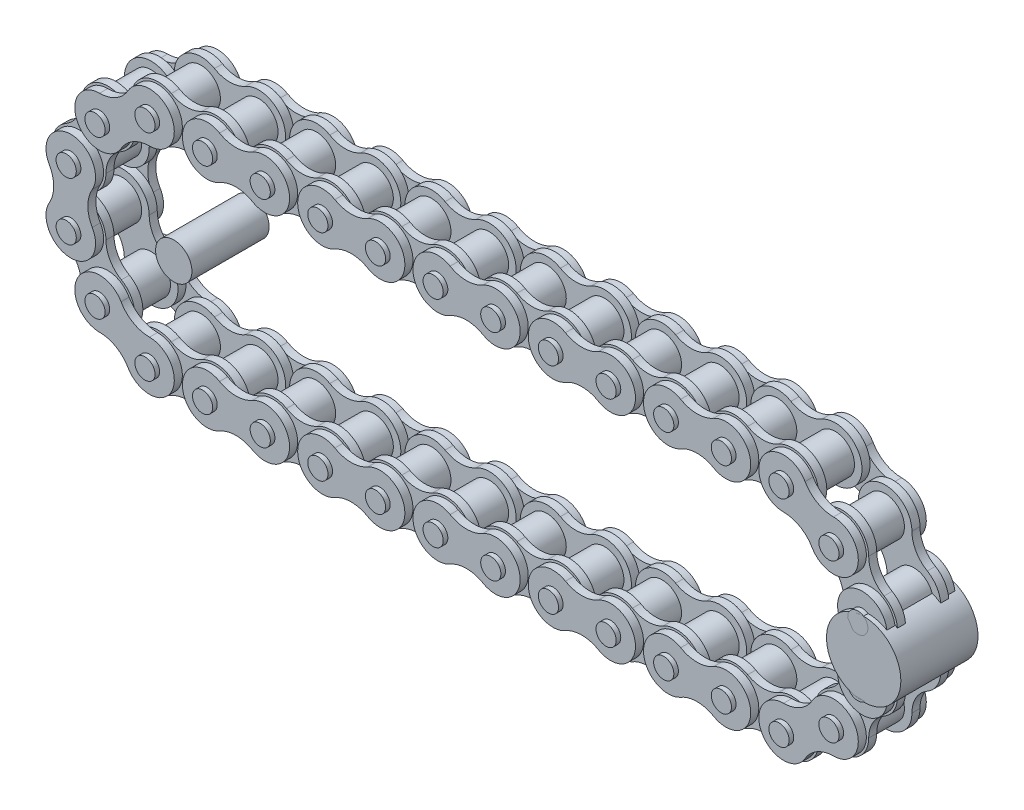
SolidWorks part; units mm, degrees
ref_plane "前视基准面" through (0, 0, 0) normal (0, 0, 1) x (1, 0, 0)
ref_plane "上视基准面" through (0, 0, 0) normal (0, 1, 0) x (1, 0, 0)
ref_plane "右视基准面" through (0, 0, 0) normal (1, 0, 0) x (0, 0, -1)
sketch "草图1" plane through (0, 0, 0) normal (0, 0, 1) x (1, 0, 0)
  circle A0 centre (-23.6985, 6.35) radius 2.225
  circle A1 centre (-23.6985, -6.35) radius 2.225
  circle A2 centre (150.6985, 6.35) radius 2.225
  circle A3 centre (150.6985, -6.35) radius 2.225
  circle A4 centre (-17.3485, 17.3485) radius 2.225
  circle A5 centre (-17.3485, -17.3485) radius 2.225
  circle A6 centre (-6.35, 23.6985) radius 2.225
  circle A7 centre (-6.35, -23.6985) radius 2.225
  circle A8 centre (144.3485, 17.3485) radius 2.225
  circle A9 centre (144.3485, -17.3485) radius 2.225
  circle A10 centre (133.35, 23.6985) radius 2.225
  circle A11 centre (133.35, -23.6985) radius 2.225
  circle A12 centre (6.35, 23.6985) radius 2.225
  circle A13 centre (6.35, -23.6985) radius 2.225
  circle A14 centre (19.05, 23.6985) radius 2.225
  circle A15 centre (19.05, -23.6985) radius 2.225
  circle A16 centre (31.75, 23.6985) radius 2.225
  circle A17 centre (31.75, -23.6985) radius 2.225
  circle A18 centre (44.45, 23.6985) radius 2.225
  circle A19 centre (44.45, -23.6985) radius 2.225
  circle A20 centre (57.15, 23.6985) radius 2.225
  circle A21 centre (57.15, -23.6985) radius 2.225
  circle A22 centre (69.85, 23.6985) radius 2.225
  circle A23 centre (69.85, -23.6985) radius 2.225
  circle A24 centre (82.55, 23.6985) radius 2.225
  circle A25 centre (82.55, -23.6985) radius 2.225
  circle A26 centre (95.25, 23.6985) radius 2.225
  circle A27 centre (95.25, -23.6985) radius 2.225
  circle A28 centre (107.95, 23.6985) radius 2.225
  circle A29 centre (107.95, -23.6985) radius 2.225
  circle A30 centre (120.65, 23.6985) radius 2.225
  circle A31 centre (120.65, -23.6985) radius 2.225
extrude "凸台-拉伸1" add sketch "草图1" along normal blind 8.5 and the other way blind 8.5
sketch "草图2" plane through (0, 0, 0) normal (0, 0, 1) x (1, 0, 0)
  circle A0 centre (-23.6985, 6.35) radius 4.255
  circle A1 centre (-23.6985, -6.35) radius 4.255
  circle A2 centre (150.6985, 6.35) radius 4.255
  circle A3 centre (150.6985, -6.35) radius 4.255
  circle A4 centre (-17.3485, 17.3485) radius 4.255
  circle A5 centre (-17.3485, -17.3485) radius 4.255
  circle A6 centre (-6.35, 23.6985) radius 4.255
  circle A7 centre (-6.35, -23.6985) radius 4.255
  circle A8 centre (144.3485, 17.3485) radius 4.255
  circle A9 centre (144.3485, -17.3485) radius 4.255
  circle A10 centre (133.35, 23.6985) radius 4.255
  circle A11 centre (133.35, -23.6985) radius 4.255
  circle A12 centre (6.35, 23.6985) radius 4.255
  circle A13 centre (6.35, -23.6985) radius 4.255
  circle A14 centre (19.05, 23.6985) radius 4.255
  circle A15 centre (19.05, -23.6985) radius 4.255
  circle A16 centre (31.75, 23.6985) radius 4.255
  circle A17 centre (31.75, -23.6985) radius 4.255
  circle A18 centre (44.45, 23.6985) radius 4.255
  circle A19 centre (44.45, -23.6985) radius 4.255
  circle A20 centre (57.15, 23.6985) radius 4.255
  circle A21 centre (57.15, -23.6985) radius 4.255
  circle A22 centre (69.85, 23.6985) radius 4.255
  circle A23 centre (69.85, -23.6985) radius 4.255
  circle A24 centre (82.55, 23.6985) radius 4.255
  circle A25 centre (82.55, -23.6985) radius 4.255
  circle A26 centre (95.25, 23.6985) radius 4.255
  circle A27 centre (95.25, -23.6985) radius 4.255
  circle A28 centre (107.95, 23.6985) radius 4.255
  circle A29 centre (107.95, -23.6985) radius 4.255
  circle A30 centre (120.65, 23.6985) radius 4.255
  circle A31 centre (120.65, -23.6985) radius 4.255
extrude "凸台-拉伸2" add sketch "草图2" along normal blind 3.875 and the other way blind 3.875
ref_plane "基准面1" through (0, 0, 3.875) normal (0, 0, 1) x (1, 0, 0)
sketch "草图3" plane through (0, 0, 3.875) normal (0, 0, 1) x (1, 0, 0)
  circle A0 centre (-23.6985, 6.35) radius 5.905
  circle A1 centre (-23.6985, -6.35) radius 5.905
  circle A2 centre (150.6985, 6.35) radius 5.905
  circle A3 centre (150.6985, -6.35) radius 5.905
  circle A4 centre (-17.3485, 17.3485) radius 5.905
  circle A5 centre (-17.3485, -17.3485) radius 5.905
  circle A6 centre (-6.35, 23.6985) radius 5.905
  circle A7 centre (-6.35, -23.6985) radius 5.905
  circle A8 centre (144.3485, 17.3485) radius 5.905
  circle A9 centre (144.3485, -17.3485) radius 5.905
  circle A10 centre (133.35, 23.6985) radius 5.905
  circle A11 centre (133.35, -23.6985) radius 5.905
  circle A12 centre (6.35, 23.6985) radius 5.905
  circle A13 centre (6.35, -23.6985) radius 5.905
  circle A14 centre (19.05, 23.6985) radius 5.905
  circle A15 centre (19.05, -23.6985) radius 5.905
  circle A16 centre (31.75, 23.6985) radius 5.905
  circle A17 centre (31.75, -23.6985) radius 5.905
  circle A18 centre (44.45, 23.6985) radius 5.905
  circle A19 centre (44.45, -23.6985) radius 5.905
  circle A20 centre (57.15, 23.6985) radius 5.905
  circle A21 centre (57.15, -23.6985) radius 5.905
  circle A22 centre (69.85, 23.6985) radius 5.905
  circle A23 centre (69.85, -23.6985) radius 5.905
  circle A24 centre (82.55, 23.6985) radius 5.905
  circle A25 centre (82.55, -23.6985) radius 5.905
  circle A26 centre (95.25, 23.6985) radius 5.905
  circle A27 centre (95.25, -23.6985) radius 5.905
  circle A28 centre (107.95, 23.6985) radius 5.905
  circle A29 centre (107.95, -23.6985) radius 5.905
  circle A30 centre (120.65, 23.6985) radius 5.905
  circle A31 centre (120.65, -23.6985) radius 5.905
extrude "凸台-拉伸3" add sketch "草图3" along normal blind 1.775
sketch "草图4" plane through (0, 0, 3.875) normal (0, 0, 1) x (1, 0, 0)
  line L0 (-26.651, 11.4639) -> (-17.7935, 6.35)
  line L1 (-23.2535, 17.3485) -> (-14.396, 12.2346)
  line L2 (-26.651, -11.4639) -> (-17.7935, -6.35)
  line L3 (-23.2535, -17.3485) -> (-14.396, -12.2346)
  line L4 (153.651, 11.4639) -> (144.7935, 6.35)
  line L5 (150.2535, 17.3485) -> (141.396, 12.2346)
  line L6 (153.651, -11.4639) -> (144.7935, -6.35)
  line L7 (150.2535, -17.3485) -> (141.396, -12.2346)
  line L8 (-3.3975, 28.8124) -> (-3.3975, 18.5846)
  line L9 (3.3975, 28.8124) -> (3.3975, 18.5846)
  line L10 (-3.3975, -28.8124) -> (-3.3975, -18.5846)
  line L11 (3.3975, -28.8124) -> (3.3975, -18.5846)
  line L12 (22.0025, 28.8124) -> (22.0025, 18.5846)
  line L13 (28.7975, 28.8124) -> (28.7975, 18.5846)
  line L14 (22.0025, -28.8124) -> (22.0025, -18.5846)
  line L15 (28.7975, -28.8124) -> (28.7975, -18.5846)
  line L16 (47.4025, 28.8124) -> (47.4025, 18.5846)
  line L17 (54.1975, 28.8124) -> (54.1975, 18.5846)
  line L18 (47.4025, -28.8124) -> (47.4025, -18.5846)
  line L19 (54.1975, -28.8124) -> (54.1975, -18.5846)
  line L20 (72.8025, 28.8124) -> (72.8025, 18.5846)
  line L21 (79.5975, 28.8124) -> (79.5975, 18.5846)
  line L22 (72.8025, -28.8124) -> (72.8025, -18.5846)
  line L23 (79.5975, -28.8124) -> (79.5975, -18.5846)
  line L24 (98.2025, 28.8124) -> (98.2025, 18.5846)
  line L25 (104.9975, 28.8124) -> (104.9975, 18.5846)
  line L26 (98.2025, -28.8124) -> (98.2025, -18.5846)
  line L27 (104.9975, -28.8124) -> (104.9975, -18.5846)
  line L28 (123.6025, 28.8124) -> (123.6025, 18.5846)
  line L29 (130.3975, 28.8124) -> (130.3975, 18.5846)
  line L30 (123.6025, -28.8124) -> (123.6025, -18.5846)
  line L31 (130.3975, -28.8124) -> (130.3975, -18.5846)
  arc A0 (-26.651, 11.4639) -> (-23.2535, 17.3485) centre (-30.0485, 17.3485) ccw
  arc A1 (-17.7935, 6.35) -> (-14.396, 12.2346) centre (-10.9985, 6.35) cw
  arc A2 (-26.651, -11.4639) -> (-23.2535, -17.3485) centre (-30.0485, -17.3485) cw
  arc A3 (-17.7935, -6.35) -> (-14.396, -12.2346) centre (-10.9985, -6.35) ccw
  arc A4 (153.651, 11.4639) -> (150.2535, 17.3485) centre (157.0485, 17.3485) cw
  arc A5 (144.7935, 6.35) -> (141.396, 12.2346) centre (137.9985, 6.35) ccw
  arc A6 (153.651, -11.4639) -> (150.2535, -17.3485) centre (157.0485, -17.3485) ccw
  arc A7 (144.7935, -6.35) -> (141.396, -12.2346) centre (137.9985, -6.35) cw
  arc A8 (-3.3975, 28.8124) -> (3.3975, 28.8124) centre (0, 34.697) ccw
  arc A9 (-3.3975, 18.5846) -> (3.3975, 18.5846) centre (0, 12.7) cw
  arc A10 (-3.3975, -28.8124) -> (3.3975, -28.8124) centre (0, -34.697) cw
  arc A11 (-3.3975, -18.5846) -> (3.3975, -18.5846) centre (0, -12.7) ccw
  arc A12 (22.0025, 28.8124) -> (28.7975, 28.8124) centre (25.4, 34.697) ccw
  arc A13 (22.0025, 18.5846) -> (28.7975, 18.5846) centre (25.4, 12.7) cw
  arc A14 (22.0025, -28.8124) -> (28.7975, -28.8124) centre (25.4, -34.697) cw
  arc A15 (22.0025, -18.5846) -> (28.7975, -18.5846) centre (25.4, -12.7) ccw
  arc A16 (47.4025, 28.8124) -> (54.1975, 28.8124) centre (50.8, 34.697) ccw
  arc A17 (47.4025, 18.5846) -> (54.1975, 18.5846) centre (50.8, 12.7) cw
  arc A18 (47.4025, -28.8124) -> (54.1975, -28.8124) centre (50.8, -34.697) cw
  arc A19 (47.4025, -18.5846) -> (54.1975, -18.5846) centre (50.8, -12.7) ccw
  arc A20 (72.8025, 28.8124) -> (79.5975, 28.8124) centre (76.2, 34.697) ccw
  arc A21 (72.8025, 18.5846) -> (79.5975, 18.5846) centre (76.2, 12.7) cw
  arc A22 (72.8025, -28.8124) -> (79.5975, -28.8124) centre (76.2, -34.697) cw
  arc A23 (72.8025, -18.5846) -> (79.5975, -18.5846) centre (76.2, -12.7) ccw
  arc A24 (98.2025, 28.8124) -> (104.9975, 28.8124) centre (101.6, 34.697) ccw
  arc A25 (98.2025, 18.5846) -> (104.9975, 18.5846) centre (101.6, 12.7) cw
  arc A26 (98.2025, -28.8124) -> (104.9975, -28.8124) centre (101.6, -34.697) cw
  arc A27 (98.2025, -18.5846) -> (104.9975, -18.5846) centre (101.6, -12.7) ccw
  arc A28 (123.6025, 28.8124) -> (130.3975, 28.8124) centre (127, 34.697) ccw
  arc A29 (123.6025, 18.5846) -> (130.3975, 18.5846) centre (127, 12.7) cw
  arc A30 (123.6025, -28.8124) -> (130.3975, -28.8124) centre (127, -34.697) cw
  arc A31 (123.6025, -18.5846) -> (130.3975, -18.5846) centre (127, -12.7) ccw
extrude "凸台-拉伸4" add sketch "草图4" along normal blind 1.775
sketch "草图5" plane through (0, 0, 3.875) normal (0, 0, 1) x (1, 0, 0)
  circle A0 centre (-23.6985, 6.35) radius 5.46
  circle A1 centre (-23.6985, -6.35) radius 5.46
  circle A2 centre (150.6985, 6.35) radius 5.46
  circle A3 centre (150.6985, -6.35) radius 5.46
  circle A4 centre (-17.3485, 17.3485) radius 5.46
  circle A5 centre (-17.3485, -17.3485) radius 5.46
  circle A6 centre (-6.35, 23.6985) radius 5.46
  circle A7 centre (-6.35, -23.6985) radius 5.46
  circle A8 centre (144.3485, 17.3485) radius 5.46
  circle A9 centre (144.3485, -17.3485) radius 5.46
  circle A10 centre (133.35, 23.6985) radius 5.46
  circle A11 centre (133.35, -23.6985) radius 5.46
  circle A12 centre (6.35, 23.6985) radius 5.46
  circle A13 centre (6.35, -23.6985) radius 5.46
  circle A14 centre (19.05, 23.6985) radius 5.46
  circle A15 centre (19.05, -23.6985) radius 5.46
  circle A16 centre (31.75, 23.6985) radius 5.46
  circle A17 centre (31.75, -23.6985) radius 5.46
  circle A18 centre (44.45, 23.6985) radius 5.46
  circle A19 centre (44.45, -23.6985) radius 5.46
  circle A20 centre (57.15, 23.6985) radius 5.46
  circle A21 centre (57.15, -23.6985) radius 5.46
  circle A22 centre (69.85, 23.6985) radius 5.46
  circle A23 centre (69.85, -23.6985) radius 5.46
  circle A24 centre (82.55, 23.6985) radius 5.46
  circle A25 centre (82.55, -23.6985) radius 5.46
  circle A26 centre (95.25, 23.6985) radius 5.46
  circle A27 centre (95.25, -23.6985) radius 5.46
  circle A28 centre (107.95, 23.6985) radius 5.46
  circle A29 centre (107.95, -23.6985) radius 5.46
  circle A30 centre (120.65, 23.6985) radius 5.46
  circle A31 centre (120.65, -23.6985) radius 5.46
extrude "凸台-拉伸5" add sketch "草图5" along normal blind 1.775 from offset 1.84
sketch "草图6" plane through (0, 0, 3.875) normal (0, 0, 1) x (1, 0, 0)
  line L0 (-28.427, 3.62) -> (-18.97, 3.62)
  line L1 (-28.427, -3.62) -> (-18.97, -3.62)
  line L2 (155.427, 3.62) -> (145.97, 3.62)
  line L3 (155.427, -3.62) -> (145.97, -3.62)
  line L4 (-17.3485, 22.8085) -> (-12.62, 14.6185)
  line L5 (-11.0785, 26.4285) -> (-6.35, 18.2385)
  line L6 (-17.3485, -22.8085) -> (-12.62, -14.6185)
  line L7 (-11.0785, -26.4285) -> (-6.35, -18.2385)
  line L8 (144.3485, 22.8085) -> (139.62, 14.6185)
  line L9 (138.0785, 26.4285) -> (133.35, 18.2385)
  line L10 (144.3485, -22.8085) -> (139.62, -14.6185)
  line L11 (138.0785, -26.4285) -> (133.35, -18.2385)
  line L12 (9.08, 28.427) -> (9.08, 18.97)
  line L13 (16.32, 28.427) -> (16.32, 18.97)
  line L14 (9.08, -28.427) -> (9.08, -18.97)
  line L15 (16.32, -28.427) -> (16.32, -18.97)
  line L16 (34.48, 28.427) -> (34.48, 18.97)
  line L17 (41.72, 28.427) -> (41.72, 18.97)
  line L18 (34.48, -28.427) -> (34.48, -18.97)
  line L19 (41.72, -28.427) -> (41.72, -18.97)
  line L20 (59.88, 28.427) -> (59.88, 18.97)
  line L21 (67.12, 28.427) -> (67.12, 18.97)
  line L22 (59.88, -28.427) -> (59.88, -18.97)
  line L23 (67.12, -28.427) -> (67.12, -18.97)
  line L24 (85.28, 28.427) -> (85.28, 18.97)
  line L25 (92.52, 28.427) -> (92.52, 18.97)
  line L26 (85.28, -28.427) -> (85.28, -18.97)
  line L27 (92.52, -28.427) -> (92.52, -18.97)
  line L28 (110.68, 28.427) -> (110.68, 18.97)
  line L29 (117.92, 28.427) -> (117.92, 18.97)
  line L30 (110.68, -28.427) -> (110.68, -18.97)
  line L31 (117.92, -28.427) -> (117.92, -18.97)
  arc A0 (-28.427, 3.62) -> (-28.427, -3.62) centre (-34.697, 0) cw
  arc A1 (-18.97, 3.62) -> (-18.97, -3.62) centre (-12.7, 0) ccw
  arc A2 (155.427, 3.62) -> (155.427, -3.62) centre (161.697, 0) ccw
  arc A3 (145.97, 3.62) -> (145.97, -3.62) centre (139.7, 0) cw
  arc A4 (-17.3485, 22.8085) -> (-11.0785, 26.4285) centre (-17.3485, 30.0485) ccw
  arc A5 (-12.62, 14.6185) -> (-6.35, 18.2385) centre (-6.35, 10.9985) cw
  arc A6 (-17.3485, -22.8085) -> (-11.0785, -26.4285) centre (-17.3485, -30.0485) cw
  arc A7 (-12.62, -14.6185) -> (-6.35, -18.2385) centre (-6.35, -10.9985) ccw
  arc A8 (144.3485, 22.8085) -> (138.0785, 26.4285) centre (144.3485, 30.0485) cw
  arc A9 (139.62, 14.6185) -> (133.35, 18.2385) centre (133.35, 10.9985) ccw
  arc A10 (144.3485, -22.8085) -> (138.0785, -26.4285) centre (144.3485, -30.0485) ccw
  arc A11 (139.62, -14.6185) -> (133.35, -18.2385) centre (133.35, -10.9985) cw
  arc A12 (9.08, 28.427) -> (16.32, 28.427) centre (12.7, 34.697) ccw
  arc A13 (9.08, 18.97) -> (16.32, 18.97) centre (12.7, 12.7) cw
  arc A14 (9.08, -28.427) -> (16.32, -28.427) centre (12.7, -34.697) cw
  arc A15 (9.08, -18.97) -> (16.32, -18.97) centre (12.7, -12.7) ccw
  arc A16 (34.48, 28.427) -> (41.72, 28.427) centre (38.1, 34.697) ccw
  arc A17 (34.48, 18.97) -> (41.72, 18.97) centre (38.1, 12.7) cw
  arc A18 (34.48, -28.427) -> (41.72, -28.427) centre (38.1, -34.697) cw
  arc A19 (34.48, -18.97) -> (41.72, -18.97) centre (38.1, -12.7) ccw
  arc A20 (59.88, 28.427) -> (67.12, 28.427) centre (63.5, 34.697) ccw
  arc A21 (59.88, 18.97) -> (67.12, 18.97) centre (63.5, 12.7) cw
  arc A22 (59.88, -28.427) -> (67.12, -28.427) centre (63.5, -34.697) cw
  arc A23 (59.88, -18.97) -> (67.12, -18.97) centre (63.5, -12.7) ccw
  arc A24 (85.28, 28.427) -> (92.52, 28.427) centre (88.9, 34.697) ccw
  arc A25 (85.28, 18.97) -> (92.52, 18.97) centre (88.9, 12.7) cw
  arc A26 (85.28, -28.427) -> (92.52, -28.427) centre (88.9, -34.697) cw
  arc A27 (85.28, -18.97) -> (92.52, -18.97) centre (88.9, -12.7) ccw
  arc A28 (110.68, 28.427) -> (117.92, 28.427) centre (114.3, 34.697) ccw
  arc A29 (110.68, 18.97) -> (117.92, 18.97) centre (114.3, 12.7) cw
  arc A30 (110.68, -28.427) -> (117.92, -28.427) centre (114.3, -34.697) cw
  arc A31 (110.68, -18.97) -> (117.92, -18.97) centre (114.3, -12.7) ccw
extrude "凸台-拉伸6" add sketch "草图6" along normal blind 1.775 from offset 1.84
mirror "镜向1" about plane through (0, 0, 0) normal (0, 0, 1) of "凸台-拉伸6", "凸台-拉伸5", "凸台-拉伸4", "凸台-拉伸3"
sketch "草图7" plane through (0, 0, 8.5) normal (0, 0, 1) x (1, 0, 0)
  line L0 (0, 0) -> (152, 0) construction
  circle A0 centre (0, 0) radius 4.006
  circle A1 centre (152, 0) radius 8.1892
  dimension "D1" = 152
extrude "凸台-拉伸7" add sketch "草图7" against normal up to surface (17 mm away) separate body up to face at (-4.125, 23.6985, -8.5)
